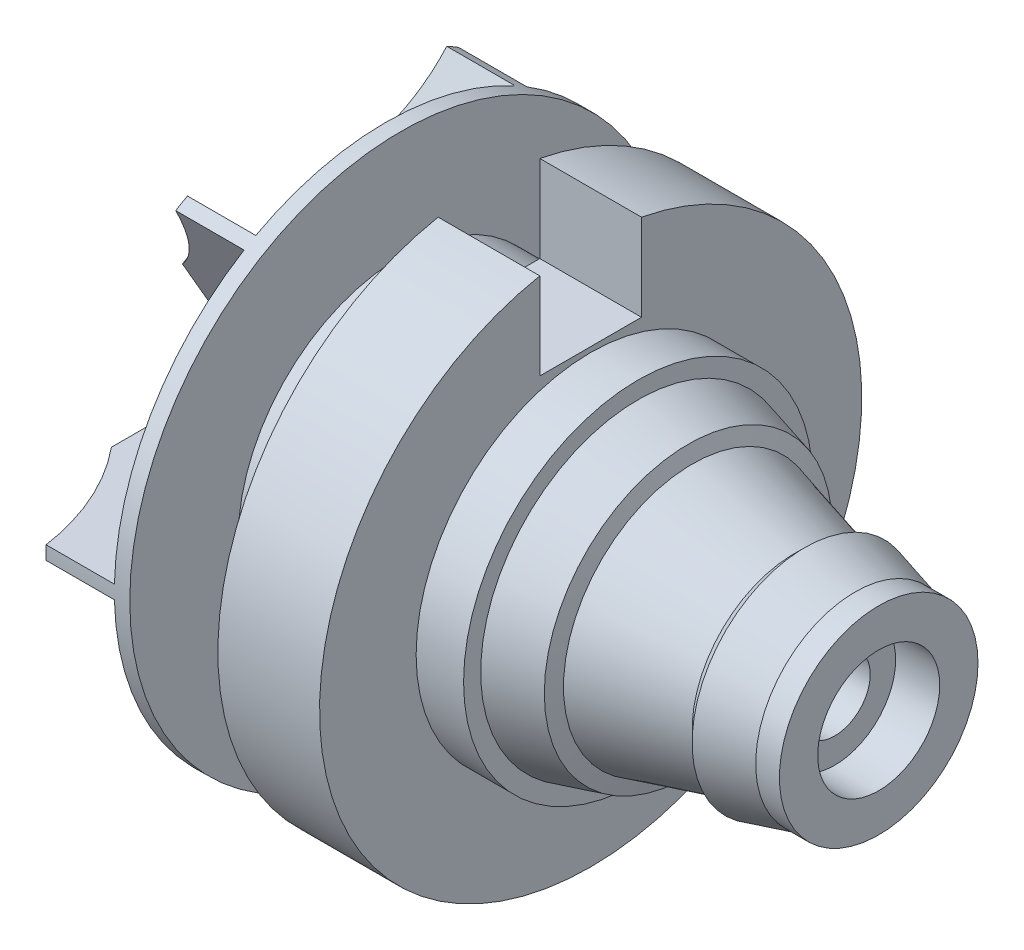
from build123d import *
from build123d.topology import SkipClean

# Parameters (mm, degrees)
M12X1_5_TAPPED_HOLE1_D     = 10.5
M12X1_5_TAPPED_HOLE1_DEPTH = 20
M12X1_5_TAPPED_HOLE1_TIP   = 3.15451825
CUT_EXTRUDE1_DEPTH         = 81.661329124
BOSS_EXTRUDE1_REACH        = 108.725
SKETCH6_R                  = 35


with BuildPart() as part:
    # Sketch1 → Revolve1 (revolve)
    with BuildSketch(Plane.XY, mode=Mode.PRIVATE) as revolve1_sk:
        with BuildLine():
            Line((-6.5, 0), (-90.5, 0))
            Line((-90.5, 0), (-90.5, 9))
            ThreePointArc((-90.5, 9), (-78.432899341, 22.667027827), (-72.77864045, 40))
            Line((-72.77864045, 40), (-70.5, 40))
            Line((-70.5, 40), (-70.5, 24))
            Line((-70.5, 24), (-57.5, 24))
            Line((-57.5, 24), (-57.5, 40))
            Line((-57.5, 40), (-42.5, 40))
            Line((-42.5, 40), (-42.5, 25.75))
            Line((-42.5, 25.75), (-35.5, 25.75))
            Line((-35.5, 25.75), (-35.5, 23.224374158))
            Line((-35.5, 23.224374158), (-28.1, 21.241550134))
            Line((-28.1, 21.241550134), (-27.502283019, 19.010839991))
            Line((-27.502283019, 19.010839991), (-12.532993162, 14.999830862))
            Line((-12.532993162, 14.999830862), (-10.9, 16.632824024))
            Line((-10.9, 16.632824024), (-3.5, 14.65))
            Line((-3.5, 14.65), (0, 14.65))
            Line((0, 14.65), (0, 9))
            Line((0, 9), (-6.5, 9))
            Line((-6.5, 9), (-6.5, 0))
        make_face()
    revolve(revolve1_sk.sketch.rotate(Axis((27.145425235, 0, 0), (-1, 0, 0)), 90), axis=Axis((27.145425235, 0, 0), (-1, 0, 0)))

    # M12x1.5 Tapped Hole1
    with Locations(Plane(origin=(-6.5, 0, 0), x_dir=(0, 0, -1), z_dir=(1, 0, 0))):
        with Locations((0, 0)):
            Hole(M12X1_5_TAPPED_HOLE1_D / 2, depth=M12X1_5_TAPPED_HOLE1_DEPTH)
            with Locations((0, 0, -(M12X1_5_TAPPED_HOLE1_DEPTH + M12X1_5_TAPPED_HOLE1_TIP / 2))):  # 118° drill point
                Cone(0, M12X1_5_TAPPED_HOLE1_D / 2, M12X1_5_TAPPED_HOLE1_TIP, mode=Mode.SUBTRACT)

    # Sketch4 → Cut-Extrude1 (cut, through all)
    with BuildSketch(Plane.ZY.offset(57.5)):
        with BuildLine():
            Line((-7.5, 39.290584114), (-7.5, 26.5))
            Line((-7.5, 26.5), (7.5, 26.5))
            Line((7.5, 26.5), (7.5, 39.290584114))
            ThreePointArc((7.5, 39.290584114), (0, 40), (-7.5, 39.290584114))
        make_face()
    extrude(amount=-CUT_EXTRUDE1_DEPTH, mode=Mode.SUBTRACT)

    # Sketch5 → Boss-Extrude1 (add, up to next)
    with BuildSketch(Plane.ZY.offset(90.5), mode=Mode.PRIVATE) as boss_extrude1_sk1:
        with BuildLine():
            ThreePointArc((20.859774427, 34.130189142), (20, 34.641016151), (19.127723619, 35.130189142))
            Line((19.127723619, 35.130189142), (3.606110551, 8.245966692))
            ThreePointArc((3.606110551, 8.245966692), (4.5, 7.794228634), (5.338161359, 7.245966692))
            Line((5.338161359, 7.245966692), (20.859774427, 34.130189142))
        make_face()
    boss_extrude1_tool1 = extrude(boss_extrude1_sk1.sketch, amount=-BOSS_EXTRUDE1_REACH, mode=Mode.PRIVATE) - part.part
    # Sketch5 → Boss-Extrude1 (add, up to next)
    with BuildSketch(Plane.ZY.offset(90.5), mode=Mode.PRIVATE) as boss_extrude1_sk2:
        with BuildLine():
            ThreePointArc((-5.338161359, 7.245966692), (-4.5, 7.794228634), (-3.606110551, 8.245966692))
            Line((-3.606110551, 8.245966692), (-19.127723619, 35.130189142))
            ThreePointArc((-19.127723619, 35.130189142), (-20, 34.641016151), (-20.859774427, 34.130189142))
            Line((-20.859774427, 34.130189142), (-5.338161359, 7.245966692))
        make_face()
    boss_extrude1_tool2 = extrude(boss_extrude1_sk2.sketch, amount=-BOSS_EXTRUDE1_REACH, mode=Mode.PRIVATE) - part.part
    # Sketch5 → Boss-Extrude1 (add, up to next)
    with BuildSketch(Plane.ZY.offset(90.5), mode=Mode.PRIVATE) as boss_extrude1_sk3:
        with BuildLine():
            Line((39.987498046, 1), (8.94427191, 1))
            ThreePointArc((8.94427191, 1), (9, 0), (8.94427191, -1))
            Line((8.94427191, -1), (39.987498046, -1))
            ThreePointArc((39.987498046, -1), (40, 0), (39.987498046, 1))
        make_face()
    boss_extrude1_tool3 = extrude(boss_extrude1_sk3.sketch, amount=-BOSS_EXTRUDE1_REACH, mode=Mode.PRIVATE) - part.part
    # Sketch5 → Boss-Extrude1 (add, up to next)
    with BuildSketch(Plane.ZY.offset(90.5), mode=Mode.PRIVATE) as boss_extrude1_sk4:
        with BuildLine():
            ThreePointArc((-8.94427191, -1), (-9, 0), (-8.94427191, 1))
            Line((-8.94427191, 1), (-39.987498046, 1))
            ThreePointArc((-39.987498046, 1), (-40, 0), (-39.987498046, -1))
            Line((-39.987498046, -1), (-8.94427191, -1))
        make_face()
    boss_extrude1_tool4 = extrude(boss_extrude1_sk4.sketch, amount=-BOSS_EXTRUDE1_REACH, mode=Mode.PRIVATE) - part.part
    # Sketch5 → Boss-Extrude1 (add, up to next)
    with BuildSketch(Plane.ZY.offset(90.5), mode=Mode.PRIVATE) as boss_extrude1_sk5:
        with BuildLine():
            Line((20.859774427, -34.130189142), (5.338161359, -7.245966692))
            ThreePointArc((5.338161359, -7.245966692), (4.5, -7.794228634), (3.606110551, -8.245966692))
            Line((3.606110551, -8.245966692), (19.127723619, -35.130189142))
            ThreePointArc((19.127723619, -35.130189142), (20, -34.641016151), (20.859774427, -34.130189142))
        make_face()
    boss_extrude1_tool5 = extrude(boss_extrude1_sk5.sketch, amount=-BOSS_EXTRUDE1_REACH, mode=Mode.PRIVATE) - part.part
    # Sketch5 → Boss-Extrude1 (add, up to next)
    with BuildSketch(Plane.ZY.offset(90.5), mode=Mode.PRIVATE) as boss_extrude1_sk6:
        with BuildLine():
            ThreePointArc((-3.606110551, -8.245966692), (-4.5, -7.794228634), (-5.338161359, -7.245966692))
            Line((-5.338161359, -7.245966692), (-20.859774427, -34.130189142))
            ThreePointArc((-20.859774427, -34.130189142), (-20, -34.641016151), (-19.127723619, -35.130189142))
            Line((-19.127723619, -35.130189142), (-3.606110551, -8.245966692))
        make_face()
    boss_extrude1_tool6 = extrude(boss_extrude1_sk6.sketch, amount=-BOSS_EXTRUDE1_REACH, mode=Mode.PRIVATE) - part.part
    add(boss_extrude1_tool1.solids().sort_by_distance((-90.5, 21.207781, 12.244318))[0])
    add(boss_extrude1_tool2.solids().sort_by_distance((-90.5, 21.207781, -12.244318))[0])
    add(boss_extrude1_tool3.solids().sort_by_distance((-90.5, 0, 24.488636))[0])
    add(boss_extrude1_tool4.solids().sort_by_distance((-90.5, 0, -24.488636))[0])
    add(boss_extrude1_tool5.solids().sort_by_distance((-90.5, -21.207781, 12.244318))[0])
    add(boss_extrude1_tool6.solids().sort_by_distance((-90.5, -21.207781, -12.244318))[0])

    # Sketch6 → Cut-Revolve1 (revolve, cut)
    with SkipClean():  # the faces are left unmerged after this step: merging them gives an invalid solid
        with BuildSketch(Plane.XY, mode=Mode.PRIVATE) as cut_revolve1_sk:
            with Locations((-117.5, 45)):
                Circle(SKETCH6_R)
        revolve(cut_revolve1_sk.sketch.rotate(Axis((-117.5, 0, 0), (1, 0, 0)), 270), axis=Axis((-117.5, 0, 0), (1, 0, 0)), mode=Mode.SUBTRACT)


solid = part.part
